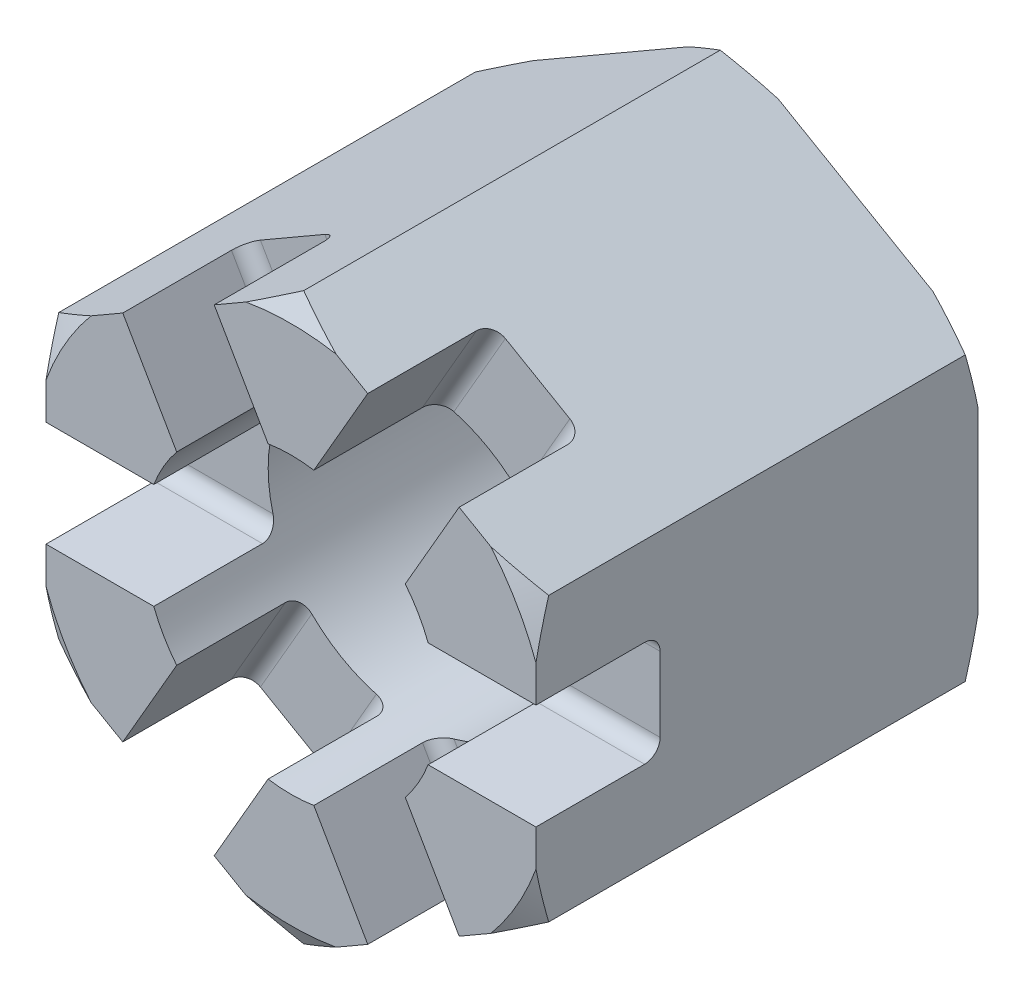
SolidWorks part; units mm, degrees
material "Q235"
ref_plane "Plane1" through (0, 0, 0) normal (0, 0, 1) x (1, 0, 0)
ref_plane "Plane2" through (0, 0, 0) normal (0, 1, 0) x (1, 0, 0)
ref_plane "Plane3" through (0, 0, 0) normal (1, 0, 0) x (0, 0, -1)
sketch "Dimension Sketch" plane through (0, 0, 0) normal (0, 0, 1) x (1, 0, 0)
  line L0 (0, 0) -> (21, 0) construction
  line L1 (22.78, 0) -> (37.88, 0) construction
  line L2 (37.88, 0) -> (57.08, 0) construction
  line L3 (-11.3333, 0) -> (2, 0) construction
  line L4 (0, 0) -> (22.78, 0) construction
  line L5 (-11.3333, 0) -> (-11.3333, 9.7) construction
  point P3 (14, 0)
  point P4 (2, 0)
  point P5 (22.78, 0)
  point P6 (17.8, 0)
  point P8 (21, 0)
  point P15 (35.58, 0)
  point P16 (42.13, 0)
  dimension "D1" = 13.3333
  dimension "D" = 14
  dimension "P" = 2
  dimension "e(min)" = 22.78
  dimension "m(max)" = 17.8
  dimension "s(max)" = 21
  dimension "da(max)" = 15.1
  dimension "dw(min)" = 19.2
  dimension "w(max)" = 12.8
  dimension "n(max)" = 4.25
  dimension "m´(min)" = 9.7
sketch "Sketch1" plane through (0, 0, 0) normal (0, 0, 1) x (1, 0, 0)
  line L0 (-9.864, 0) -> (9.864, 0) construction
  line L1 (0, 11.39) -> (0, -11.39) construction
  line L3 (0, 11.39) -> (-9.864, 5.695)
  line L4 (-9.864, 5.695) -> (-9.864, -5.695)
  line L5 (-9.864, -5.695) -> (0, -11.39)
  line L6 (0, -11.39) -> (9.864, -5.695)
  line L7 (9.864, -5.695) -> (9.864, 5.695)
  line L8 (9.864, 5.695) -> (0, 11.39)
  circle A0 centre (0, 0) radius 9.864 construction
  circle A1 centre (0, 0) radius 5.9175
  dimension "D" = 11.835
  dimension "e" = 22.78
extrude "Base-Extrude" add sketch "Sketch1" along normal blind 17.8
cosmetic thread "Cosmetic Thread1" parameters "D2"=14
sketch "Sketch2" plane through (0, 0, 0) normal (0, 0, -1) x (-1, 0, 0)
  circle A0 centre (0, 0) radius 10.5
  circle A1 centre (0, 0) radius 5.9175 construction
  dimension "s" = 21
extrude "Cut-Extrude1" cut sketch "Sketch2" against normal through all draft 60 flip side to cut
sketch "Sketch3" plane through (0, 0, 17.8) normal (0, 0, 1) x (1, 0, 0)
  circle A0 centre (0, 0) radius 10.5
  dimension "D1" = 21
extrude "Cut-Extrude2" cut sketch "Sketch3" against normal through all draft 60 flip side to cut
sketch "Sketch6" plane through (9.864, 0, 0) normal (1, 0, 0) x (0, 0, -1)
  line L0 (-14.9451, 0) -> (3.4921, 0) construction
  line L1 (-17.8, 0) -> (0, 0) construction
  line L3 (-17.8, -3.5987) -> (-17.8, 3.5987) construction
  line L4 (-17.8, -2.125) -> (-17.8, 2.125)
  line L5 (-17.8, 2.125) -> (-13.425, 2.125)
  line L6 (-12.8, -1.5) -> (-12.8, 1.5)
  line L7 (0, -3.5987) -> (0, 3.5987) construction
  line L8 (-17.8, -2.125) -> (-13.425, -2.125)
  arc A0 (-13.425, 2.125) -> (-12.8, 1.5) centre (-13.425, 1.5) cw
  arc A1 (-13.425, -2.125) -> (-12.8, -1.5) centre (-13.425, -1.5) ccw
  point P14 (-12.8, 2.125)
  point P17 (-12.8, -2.125)
  dimension "D1" = 0.625
  dimension "W" = 12.8
  dimension "n" = 2.125
extrude "Cut-Extrude3" cut sketch "Sketch6" against normal through all
pattern_circular "CirPattern1" count 3 over 360 about axis through (0, 0, 0) along (0, 0, 1) of "Cut-Extrude3"
chamfer "Chamfer1" distance 0.2208 angle 45 1 edges at (5.9175, 0, 0)
